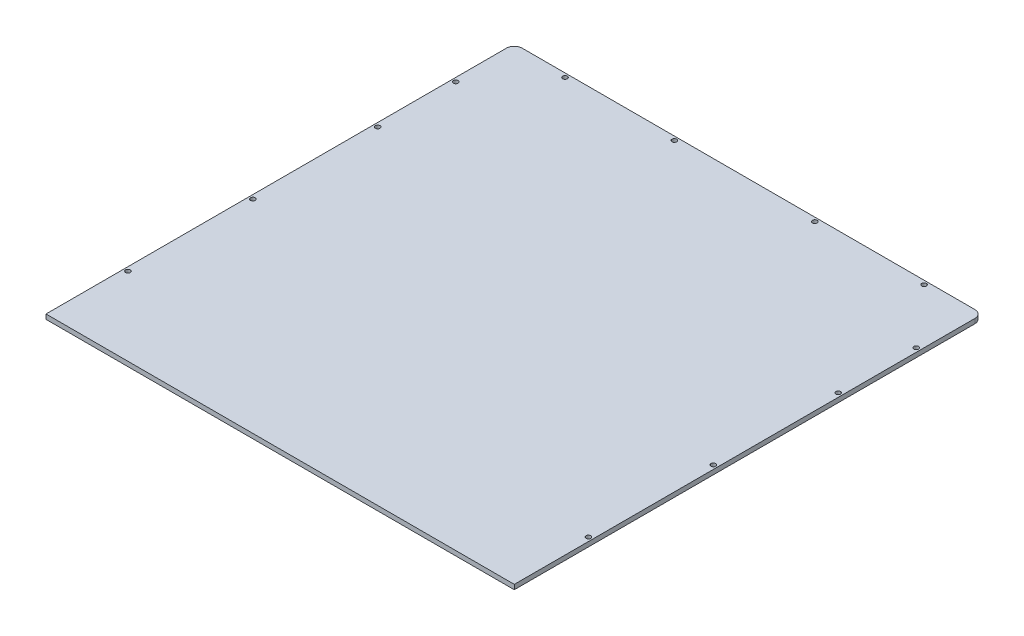
SolidWorks part; units mm, degrees
ref_plane "Front Plane" through (0, 0, 0) normal (0, 0, 1) x (1, 0, 0)
ref_plane "Top Plane" through (0, 0, 0) normal (0, 1, 0) x (1, 0, 0)
ref_plane "Right Plane" through (0, 0, 0) normal (1, 0, 0) x (0, 0, -1)
sketch "Sketch1" plane through (0, 0, 0) normal (0, 1, 0) x (1, 0, 0)
  line L0 (0, -1000) -> (0, 49000) construction
  line L1 (-150, -150) -> (150, -150)
  line L2 (-150, -150) -> (-150, 145)
  line L3 (-145, 150) -> (145, 150)
  line L4 (150, -150) -> (150, 145)
  line L5 (-150, -150) -> (150, 150) construction
  line L6 (-150, 150) -> (150, -150) construction
  arc A0 (145, 150) -> (150, 145) centre (145, 145) cw
  arc A1 (-150, 145) -> (-145, 150) centre (-145, 145) cw
  circle A2 centre (-147.5, -100) radius 1.5
  circle A3 centre (-147.5, -20) radius 1.5
  circle A4 centre (-147.5, 60) radius 1.5
  circle A5 centre (-147.5, 110) radius 1.5
  circle A6 centre (-115, 147.5) radius 1.5
  circle A7 centre (-45, 147.5) radius 1.5
  circle A8 centre (45, 147.5) radius 1.5
  circle A9 centre (115, 147.5) radius 1.5
  circle A10 centre (147.5, -20) radius 1.5
  circle A11 centre (147.5, -100) radius 1.5
  circle A12 centre (147.5, 110) radius 1.5
  circle A13 centre (147.5, 60) radius 1.5
  point P0 (0, 0)
  dimension "D3" = 5
  dimension "D4" = 3
  dimension "D5" = 2.5
  dimension "D6" = 50
  dimension "D8" = 80
  dimension "D15" = 35
  dimension "D1" = 300
  dimension "D2" = 300
  dimension "D7" = 2.5
  dimension "D9" = 80
  dimension "D10" = 50
  dimension "D11" = 2.5
  dimension "D12" = 2.5
  dimension "D13" = 2.5
  dimension "D14" = 2.5
  dimension "D16" = 70
extrude "Boss-Extrude1" add sketch "Sketch1" along normal blind 3
